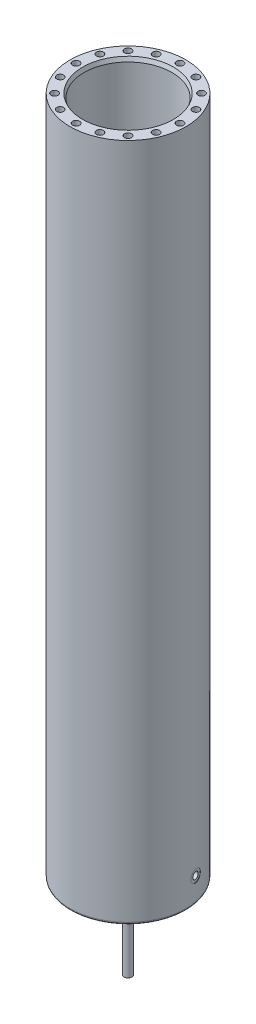
SolidWorks part; units mm, degrees
material "AISI 1045 钢，冷拔"
ref_plane "Front Plane" through (0, 0, 0) normal (0, 0, 1) x (1, 0, 0)
ref_plane "Top Plane" through (0, 0, 0) normal (0, 1, 0) x (1, 0, 0)
ref_plane "Right Plane" through (0, 0, 0) normal (1, 0, 0) x (0, 0, -1)
sketch "Sketch1" plane through (0, 0, 0) normal (0, 0, 1) x (1, 0, 0)
  line L0 (0, 0) -> (0, 106.6643) construction
  line L1 (0, 0) -> (-139, 0)
  line L2 (-145, 6) -> (-145, 1701)
  line L3 (-145, 1701) -> (-113.6397, 1701)
  line L4 (-110, 1691) -> (-110, 50)
  line L5 (-105, 45) -> (0, 45)
  line L6 (0, 45) -> (0, 0)
  line L7 (-113.6397, 1701) -> (-110, 1691)
  arc A0 (-110, 50) -> (-105, 45) centre (-105, 50) ccw
  arc A1 (-139, 0) -> (-145, 6) centre (-139, 6) cw
  point P12 (-145, 0)
  dimension "D5" = 5
  dimension "D6" = 6
  dimension "D1" = 220
  dimension "D2" = 35
  dimension "D3" = 45
  dimension "D4" = 20
  dimension "D7" = 290
  dimension "D8" = 10
  dimension "D9" = 1701
revolve "Revolve1" add sketch "Sketch1" angle 360 about L0
hole_wizard "M20 Tapped Hole1" positions "Sketch3" profile "Sketch2" tap size "M20" standard "Gb"
sketch "Sketch3" plane through (0, 1701, 0) normal (0, 1, 0) x (1, 0, 0)
  circle A0 centre (0, 0) radius 130 construction
  point P0 (-130, 0)
  point P12 (-120.1043, 49.7488)
  point P13 (-91.9239, 91.9239)
  point P14 (-49.7488, 120.1043)
  point P15 (0, 130)
  point P16 (49.7488, 120.1043)
  point P17 (91.9239, 91.9239)
  point P18 (120.1043, 49.7488)
  point P19 (130, 0)
  point P20 (120.1043, -49.7488)
  point P21 (91.9239, -91.9239)
  point P22 (49.7488, -120.1043)
  point P23 (0, -130)
  point P24 (-49.7488, -120.1043)
  point P25 (-91.9239, -91.9239)
  point P26 (-120.1043, -49.7488)
  dimension "D1" = 260
  dimension "D2" = 16
sketch "Sketch2" plane through (-130, 1701, 0) normal (1, 0, 0) x (0, 0, 1)
  line L0 (0, 0) -> (0, 62.7575)
  line L1 (0, 62.7575) -> (8.75, 57.5)
  line L2 (8.75, 57.5) -> (8.75, 0)
  line L5 (8.75, 0) -> (0, 0)
  line L10 (0, 62.7575) -> (-8.75, 57.5) construction
  line L11 (0, -6.35) -> (0, 107.95) construction
  dimension "螺纹孔钻头直径" = 17.5
  dimension "螺纹孔钻头深度" = 57.5
  dimension "导头角度" = 118
cosmetic thread "Cosmetic thread18" parameters "D1"=45, "D2"=20
cosmetic thread "Cosmetic thread19" parameters "D1"=45, "D2"=20
cosmetic thread "Cosmetic thread20" parameters "D1"=45, "D2"=20
cosmetic thread "Cosmetic thread21" parameters "D1"=45, "D2"=20
cosmetic thread "Cosmetic thread22" parameters "D1"=45, "D2"=20
cosmetic thread "Cosmetic thread23" parameters "D1"=45, "D2"=20
cosmetic thread "Cosmetic thread24" parameters "D1"=45, "D2"=20
cosmetic thread "Cosmetic thread25" parameters "D1"=45, "D2"=20
cosmetic thread "Cosmetic thread26" parameters "D1"=45, "D2"=20
cosmetic thread "Cosmetic thread27" parameters "D1"=45, "D2"=20
cosmetic thread "Cosmetic thread28" parameters "D1"=45, "D2"=20
cosmetic thread "Cosmetic thread29" parameters "D1"=45, "D2"=20
cosmetic thread "Cosmetic thread30" parameters "D1"=45, "D2"=20
cosmetic thread "Cosmetic thread31" parameters "D1"=45, "D2"=20
cosmetic thread "Cosmetic thread32" parameters "D1"=45, "D2"=20
cosmetic thread "Cosmetic thread33" parameters "D1"=45, "D2"=20
ref_plane "Plane1" through (0, 0, 0) normal (0.1908, 0, 0.9816) x (0.9816, 0, -0.1908)
hole_wizard "Hole size per socket head cap screw type1" positions "3DSketch1" profile "Sketch4" counterbore size "M10" standard "Gb"
sketch3d "3DSketch1"
  point P0 (142.3359, 62, -27.6673)
  dimension "D1" = 62
sketch "Sketch4" plane through (142.3359, 62, -27.6673) normal (0, 1, 0) x (-0.1908, 0, -0.9816)
  line L0 (0, 0) -> (0, 53.6052)
  line L1 (0, 53.6052) -> (6, 50)
  line L2 (6, 50) -> (6, 1)
  line L3 (6, 1) -> (15, 1)
  line L4 (15, 1) -> (15, 0)
  line L5 (15, 0) -> (0, 0)
  line L10 (0, 53.6052) -> (-6, 50) construction
  line L11 (0, -6.35) -> (0, 107.95) construction
  dimension "孔直径" = 12
  dimension "孔深度" = 50
  dimension "柱形沉头孔直径" = 30
  dimension "柱形沉头孔深度" = 1
  dimension "导头角度" = 118
hole_wizard "M18x1.5 Tapped Hole1" positions "Sketch6" profile "Sketch5" tap size "M18x1.5" standard "Gb"
sketch "Sketch6" plane through (141.3543, 0, -27.4765) normal (0.9816, 0, -0.1908) x (-0.1908, 0, -0.9816)
  point P0 (0, 62)
sketch "Sketch5" plane through (141.3543, 62, -27.4765) normal (0, 1, 0) x (-0.1908, 0, -0.9816)
  line L0 (0, 0) -> (0, 32.4571)
  line L1 (0, 32.4571) -> (8.25, 27.5)
  line L2 (8.25, 27.5) -> (8.25, 0)
  line L5 (8.25, 0) -> (0, 0)
  line L10 (0, 32.4571) -> (-8.25, 27.5) construction
  line L11 (0, -6.35) -> (0, 107.95) construction
  dimension "螺纹孔钻头直径" = 16.5
  dimension "螺纹孔钻头深度" = 27.5
  dimension "导头角度" = 118
cosmetic thread "Cosmetic thread17" parameters "D1"=20, "D2"=18
sketch "Sketch7" plane through (0, 0, 0) normal (0, -1, 0) x (1, 0, 0)
  circle A0 centre (0, 0) radius 25
  dimension "D1" = 50
extrude "Boss-Extrude1" add sketch "Sketch7" along normal blind 10 separate body
sketch "Sketch8" plane through (0, -10, 0) normal (0, -1, 0) x (1, 0, 0)
  circle A0 centre (0, 0) radius 10
  dimension "D1" = 20
extrude "Boss-Extrude2" add sketch "Sketch8" along normal blind 200
